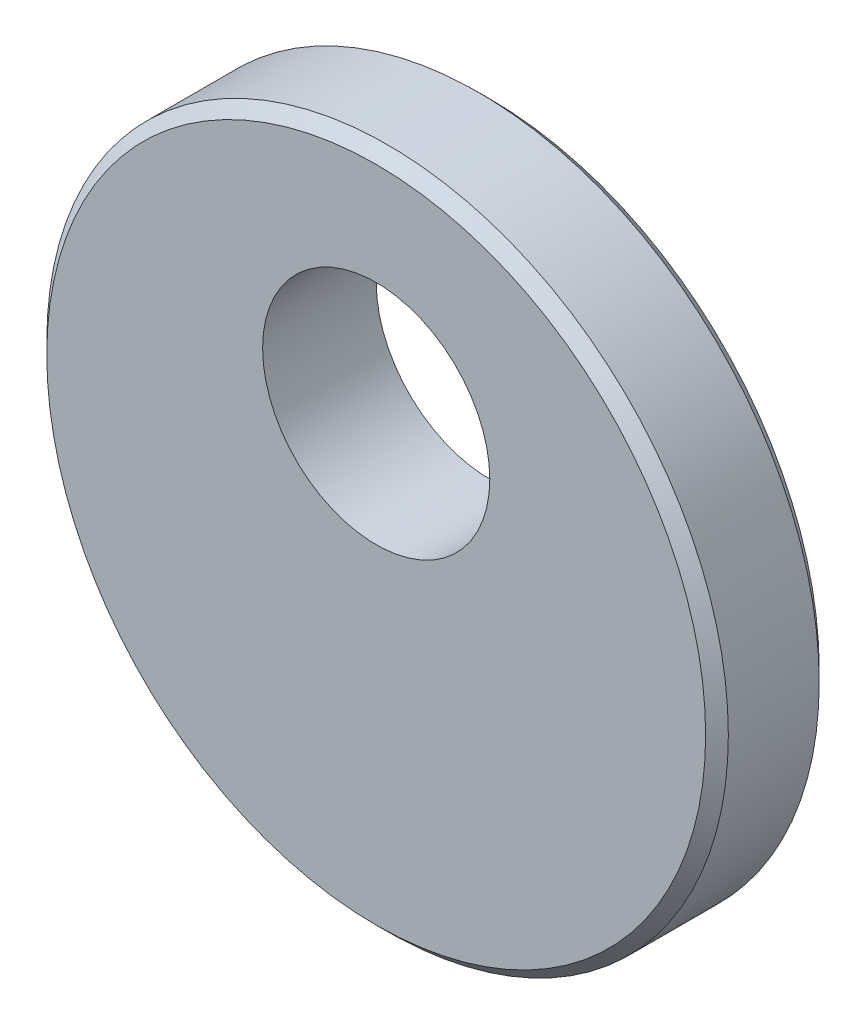
from build123d import *

# Parameters (mm, degrees)
SKETCH1_R           = 15
BOSS_EXTRUDE1_DEPTH = 5
SKETCH2_R           = 5
CUT_EXTRUDE1_DEPTH  = 5
CHAMFER1_SIZE       = 0.5


with BuildPart() as part:
    # Sketch1 → Boss-Extrude1 (new body)
    with BuildSketch(Plane.XY):
        Circle(SKETCH1_R)
    extrude(amount=BOSS_EXTRUDE1_DEPTH)

    # Sketch2 → Cut-Extrude1 (cut)
    with BuildSketch(Plane.XY.offset(5)):
        with Locations((0, 5)):
            Circle(SKETCH2_R)
    extrude(amount=-CUT_EXTRUDE1_DEPTH, mode=Mode.SUBTRACT)

    # Chamfer1
    chamfer1_edges = [part.edges().sort_by_distance(p)[0] for p in [
        (-15, 0, 0),
        (-15, 0, 5),
    ]]
    chamfer(chamfer1_edges, length=CHAMFER1_SIZE)


solid = part.part
